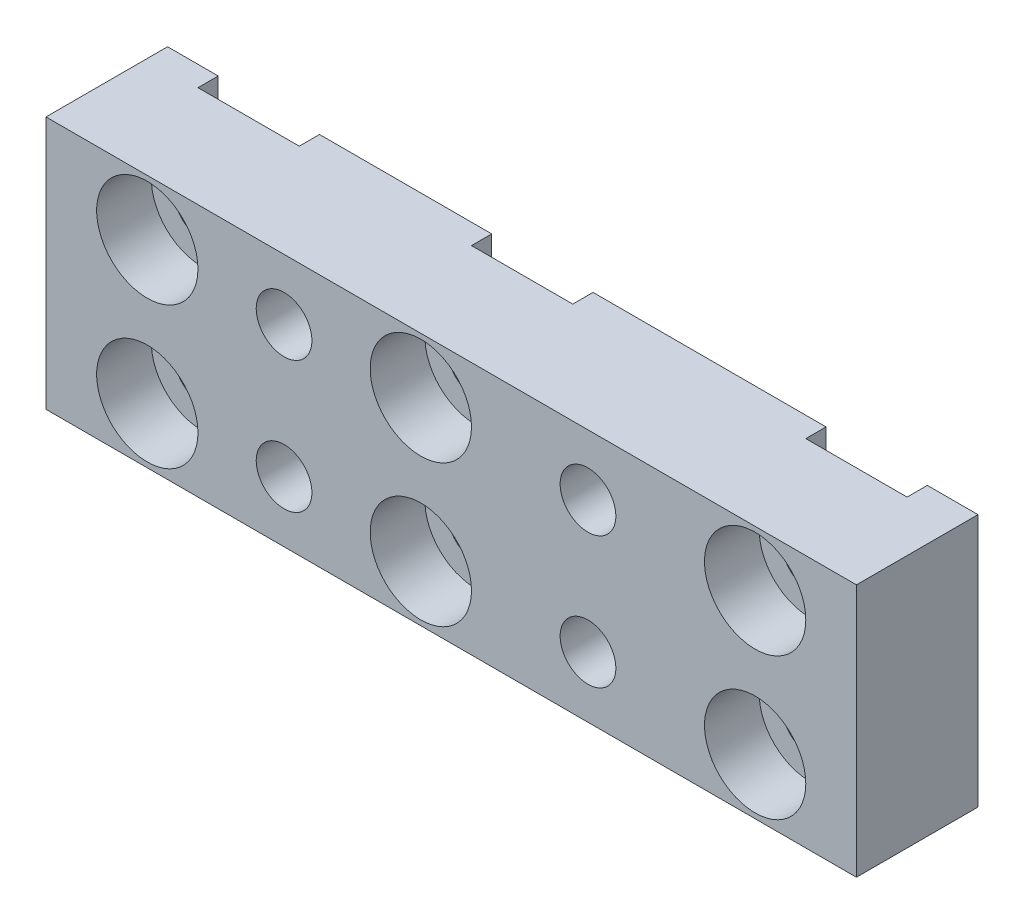
SolidWorks part; units mm, degrees
ref_plane "Front Plane" through (0, 0, 0) normal (0, 0, 1) x (1, 0, 0)
ref_plane "Top Plane" through (0, 0, 0) normal (0, 1, 0) x (1, 0, 0)
ref_plane "Right Plane" through (0, 0, 0) normal (1, 0, 0) x (0, 0, -1)
sketch "Sketch1" plane through (0, 0, 0) normal (0, 0, 1) x (1, 0, 0)
  line L1 (-40, 12.5) -> (40, 12.5)
  line L2 (-40, 12.5) -> (-40, -12.5)
  line L3 (-40, -12.5) -> (40, -12.5)
  line L4 (40, 12.5) -> (40, -12.5)
  line L5 (-40, 12.5) -> (40, -12.5) construction
  line L6 (-40, -12.5) -> (40, 12.5) construction
  point P0 (0, 0)
  dimension "D1" = 80
  dimension "D2" = 25
extrude "Boss-Extrude1" add sketch "Sketch1" along normal blind 12
sketch "Sketch2" plane through (0, 12.5, 0) normal (0, 1, 0) x (1, 0, 0)
  line L0 (40, 0) -> (-40, 0) construction
  line L1 (-35, 0) -> (-25, 0)
  line L2 (-35, 0) -> (-35, -2)
  line L3 (-35, -2) -> (-25, -2)
  line L4 (-25, 0) -> (-25, -2)
  line L5 (40, -12) -> (40, 0) construction
  line L6 (-8, 0) -> (2, 0)
  line L7 (-8, 0) -> (-8, -2)
  line L8 (-8, -2) -> (2, -2)
  line L9 (2, 0) -> (2, -2)
  line L10 (25, 0) -> (35, 0)
  line L11 (25, 0) -> (25, -2)
  line L12 (25, -2) -> (35, -2)
  line L13 (35, 0) -> (35, -2)
  dimension "D1" = 10
  dimension "D2" = 17
  dimension "D3" = 23
  dimension "D4" = 2
  dimension "D5" = 5
extrude "Cut-Extrude1" cut sketch "Sketch2" against normal through all
hole_wizard "CBORE for M5 Hex Socket Head Cap Screw1" positions "Sketch3" profile "Sketch4" counterbore size "M5" standard "ISO" end condition through all
sketch "Sketch3" plane through (0, 0, 12) normal (0, 0, 1) x (1, 0, 0)
  line L0 (0, 0) -> (8.4077, 0) construction
  line L2 (-35, -12.5) -> (-35, 12.5) construction
  line L3 (-8, -12.5) -> (-8, 12.5) construction
  line L4 (25, -12.5) -> (25, 12.5) construction
  point P0 (-30, 7)
  point P2 (-30, -7)
  point P4 (-3, 7)
  point P6 (-3, -7)
  point P8 (30, 7)
  point P10 (30, -7)
  dimension "D1" = 14
  dimension "D2" = 5
  dimension "D3" = 5
  dimension "D4" = 5
sketch "Sketch4" plane through (-30, 7, 12) normal (1, 0, 0) x (0, -1, 0)
  line L0 (0, 0) -> (0, 12)
  line L1 (0, 12) -> (2.75, 12)
  line L3 (2.75, 12) -> (2.75, 5.4)
  line L4 (2.75, 5.4) -> (5, 5.4)
  line L5 (5, 5.4) -> (5, 0)
  line L7 (5, 0) -> (0, 0)
  line L11 (0, -6.35) -> (0, 107.95) construction
  dimension "通孔孔直径" = 5.5
  dimension "通孔孔深度" = 12
  dimension "柱形沉头孔直径" = 10
  dimension "柱形沉头孔深度" = 5.4
hole_wizard "CBORE for M5 Hex Socket Head Cap Screw2" positions "Sketch5" profile "Sketch6" counterbore size "M5" standard "ISO" end condition through all
sketch "Sketch5" plane through (0, 0, 0) normal (0, 0, -1) x (-1, 0, 0)
  line L0 (-6.3274, 0) -> (0, 0) construction
  line L3 (-13.5, 12.5) -> (-13.5, 6.5) construction
  line L4 (-25, 12.5) -> (-2, 12.5) construction
  line L6 (16.5, 12.5) -> (16.5, 6.5) construction
  line L7 (8, 12.5) -> (25, 12.5) construction
  point P0 (-13.5, 6.5)
  point P2 (-13.5, -6.5)
  point P4 (16.5, 6.5)
  point P6 (16.5, -6.5)
  dimension "D1" = 6
sketch "Sketch6" plane through (13.5, 6.5, 0) normal (1, 0, 0) x (0, 1, 0)
  line L0 (0, 0) -> (0, 12)
  line L1 (0, 12) -> (2.75, 12)
  line L3 (2.75, 12) -> (2.75, 5.4)
  line L4 (2.75, 5.4) -> (5, 5.4)
  line L5 (5, 5.4) -> (5, 0)
  line L7 (5, 0) -> (0, 0)
  line L11 (0, -6.35) -> (0, 107.95) construction
  dimension "通孔孔直径" = 5.5
  dimension "通孔孔深度" = 12
  dimension "柱形沉头孔直径" = 10
  dimension "柱形沉头孔深度" = 5.4
